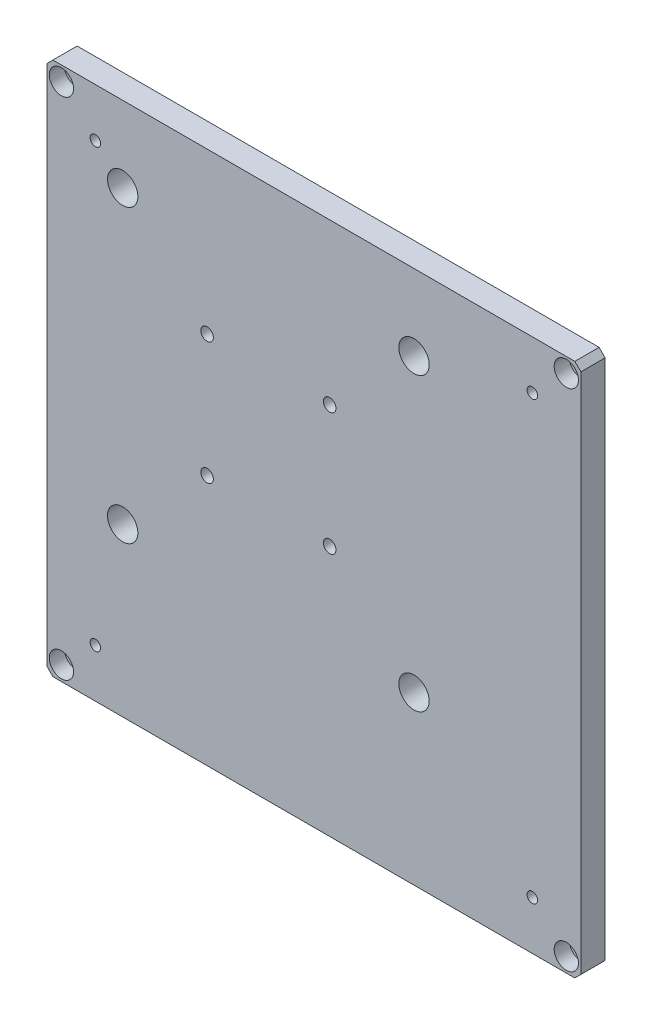
SolidWorks part; units mm, degrees
ref_plane "Front Plane" through (0, 0, 0) normal (0, 0, 1) x (1, 0, 0)
ref_plane "Top Plane" through (0, 0, 0) normal (0, 1, 0) x (1, 0, 0)
ref_plane "Right Plane" through (0, 0, 0) normal (1, 0, 0) x (0, 0, -1)
sketch "Sketch1" plane through (0, 0, 0) normal (0, 0, 1) x (1, 0, 0)
  line L0 (498.7494, 365) -> (-361.2506, 365)
  line L1 (508.7494, 355) -> (498.7494, 365)
  line L2 (508.7494, -505) -> (508.7494, 355)
  line L3 (498.7494, -515) -> (508.7494, -505)
  line L4 (-361.2506, -515) -> (498.7494, -515)
  line L5 (-371.2506, -505) -> (-361.2506, -515)
  line L6 (-371.2506, 355) -> (-371.2506, -505)
  line L7 (-361.2506, 365) -> (-371.2506, 355)
  circle A0 centre (428.7494, -435) radius 8.647
  circle A1 centre (-291.2506, 285) radius 8.647
  circle A2 centre (428.7494, 285) radius 8.647
  circle A3 centre (-291.2506, -435) radius 8.647
  circle A4 centre (484.7494, -491) radius 13
  circle A5 centre (-347.2506, 341) radius 13
  circle A6 centre (484.7494, 341) radius 13
  circle A7 centre (-347.2506, -491) radius 13
  circle A8 centre (-107.2506, -101) radius 10.376
  circle A9 centre (94.7494, 101) radius 10.376
  circle A10 centre (-107.2506, 101) radius 10.376
  circle A11 centre (94.7494, -101) radius 10.376
  circle A12 centre (-246.2506, -240) radius 25
  circle A13 centre (233.7494, 240) radius 25
  circle A14 centre (-246.2506, 240) radius 25
  circle A15 centre (233.7494, -240) radius 25
extrude "Boss-Extrude1" add sketch "Sketch1" along normal blind 40
sketch "Sketch2" plane through (0, 0, 40) normal (0, 0, 1) x (1, 0, 0)
  circle A0 centre (-347.2506, 341) radius 20
  circle A1 centre (484.7494, 341) radius 20
  circle A2 centre (484.7494, -491) radius 20
  circle A3 centre (-347.2506, -491) radius 20
  dimension "D1" = 40
extrude "Cut-Extrude1" cut sketch "Sketch2" against normal blind 25 contours A3 | A0 | A1 | A2
